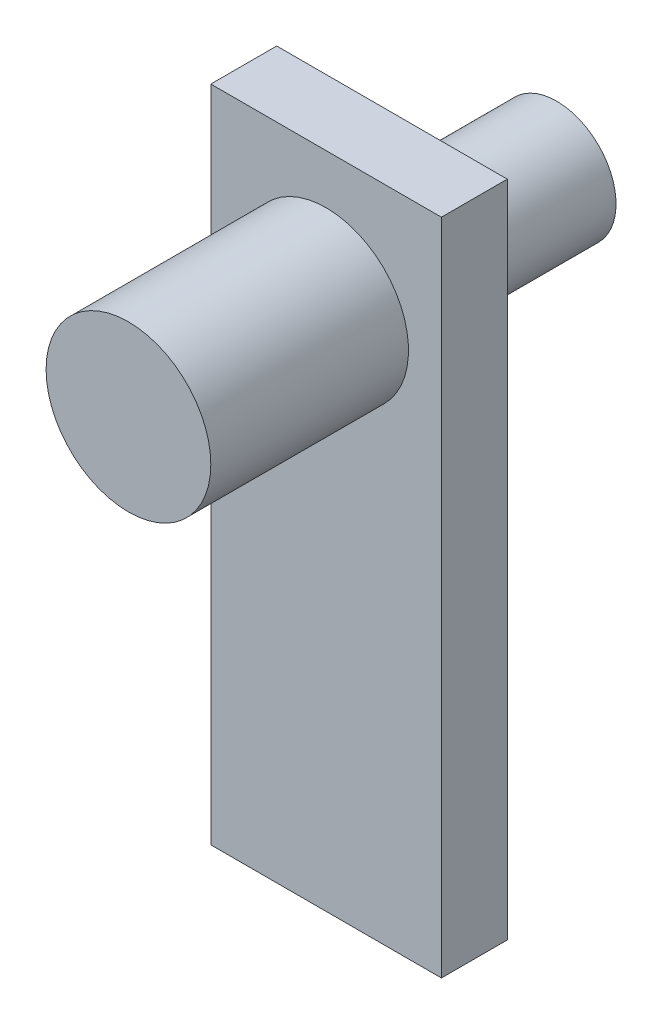
SolidWorks part; units mm, degrees
ref_plane "前视基准面" through (0, 0, 0) normal (0, 0, 1) x (1, 0, 0)
ref_plane "上视基准面" through (0, 0, 0) normal (0, 1, 0) x (1, 0, 0)
ref_plane "右视基准面" through (0, 0, 0) normal (1, 0, 0) x (0, 0, -1)
sketch "草图1" plane through (0, 0, 0) normal (0, 0, 1) x (1, 0, 0)
  line L1 (-17.5, -50) -> (17.5, -50)
  line L2 (-17.5, -50) -> (-17.5, 50)
  line L3 (-17.5, 50) -> (17.5, 50)
  line L4 (17.5, -50) -> (17.5, 50)
  line L5 (-17.5, -50) -> (17.5, 50) construction
  line L6 (-17.5, 50) -> (17.5, -50) construction
  point P0 (0, 0)
  dimension "D1" = 35
  dimension "D2" = 100
extrude "凸台-拉伸1" add sketch "草图1" along normal blind 10
sketch "草图2" plane through (0, 0, 10) normal (0, 0, 1) x (1, 0, 0)
  line L0 (0, 0) -> (0, 50) construction
  line L1 (17.5, 50) -> (-17.5, 50) construction
  circle A0 centre (0, 30) radius 12.5
  dimension "D1" = 25
  dimension "D2" = 20
extrude "凸台-拉伸2" add sketch "草图2" along normal blind 30
sketch "草图3" plane through (0, 0, 0) normal (0, 0, -1) x (-1, 0, 0)
  line L0 (0, 0) -> (0, 50) construction
  line L1 (-17.5, 50) -> (17.5, 50) construction
  circle A0 centre (0, 30) radius 9
  dimension "D1" = 18
  dimension "D2" = 20
extrude "凸台-拉伸3" add sketch "草图3" along normal blind 25
